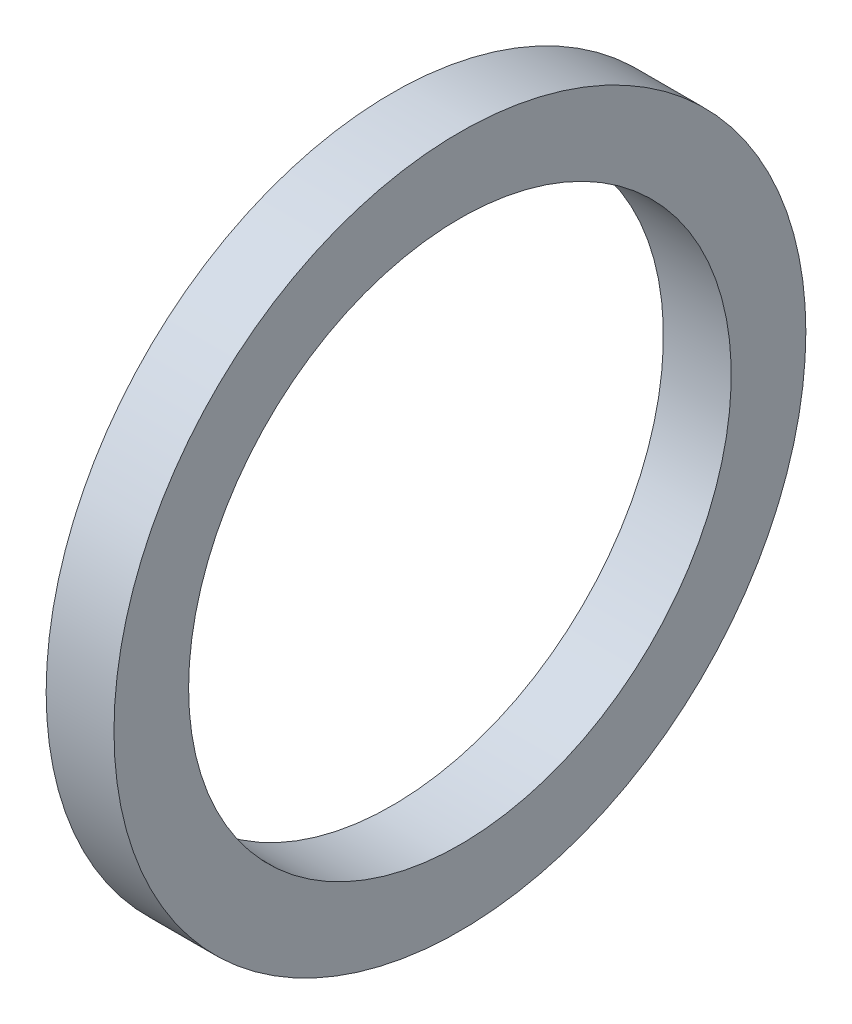
from build123d import *

# Parameters (mm, degrees)
SKETCH_1_W = 5
SKETCH_1_H = 5.5


with BuildPart() as part:
    # 草图1 → 旋转1 (revolve)
    with BuildSketch(Plane(origin=(0, 0, 0), x_dir=(1, 0, 0), z_dir=(0, 1, 0)), mode=Mode.PRIVATE) as revolve_1_sk:
        with Locations((2.5, 22.75)):
            Rectangle(SKETCH_1_W, SKETCH_1_H)
    revolve(revolve_1_sk.sketch.rotate(Axis((-329.823645462, 0, 0), (1, 0, 0)), 180), axis=Axis((-329.823645462, 0, 0), (1, 0, 0)))


solid = part.part
